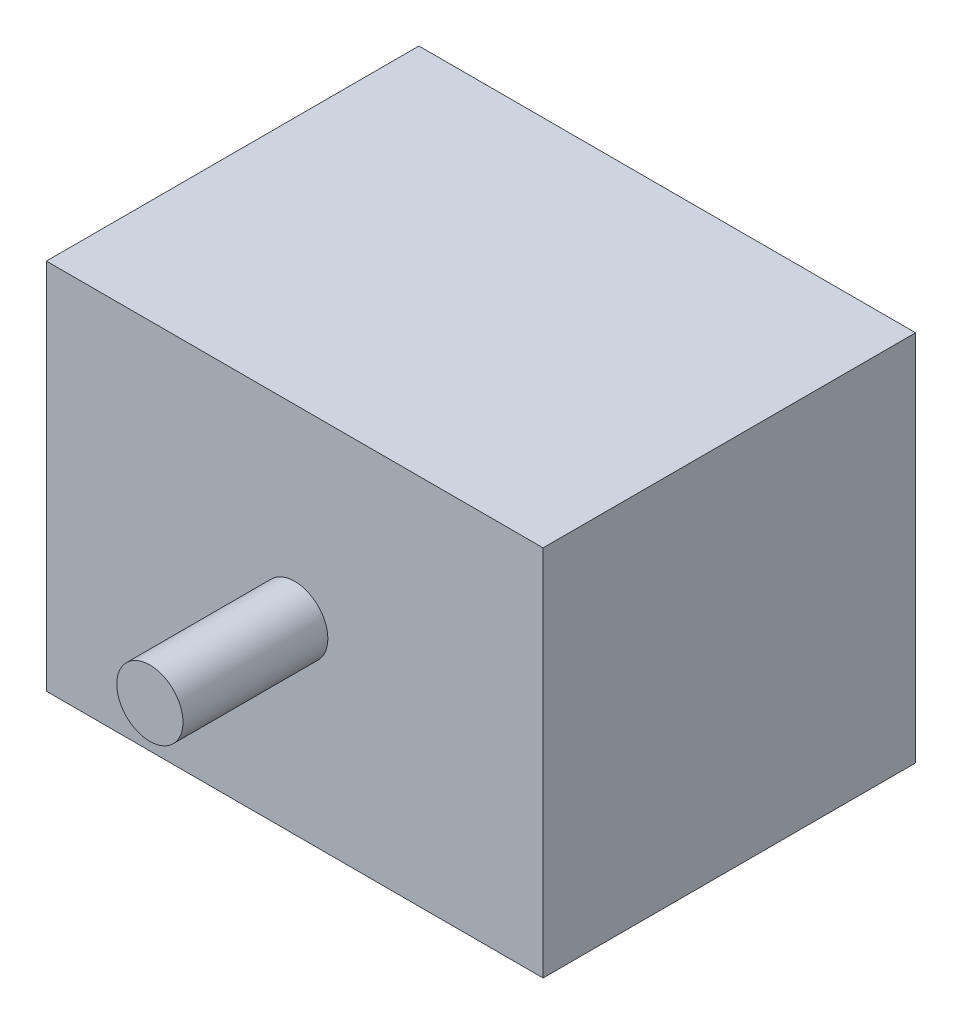
from build123d import *

# Parameters (mm, degrees)
SKETCH_1_W      = 120
SKETCH_1_H      = 90
EXTRUDE_1_DEPTH = 45
SKETCH_2_R      = 8
EXTRUDE_2_DEPTH = 80


with BuildPart() as part:
    # 草图1 → 凸台-拉伸1 (new, symmetric)
    with BuildSketch(Plane.XY):
        Rectangle(SKETCH_1_W, SKETCH_1_H)
    extrude(amount=EXTRUDE_1_DEPTH, both=True)

    # 草图2 → 凸台-拉伸2 (add, symmetric)
    with BuildSketch(Plane.XY):
        Circle(SKETCH_2_R)
    extrude(amount=EXTRUDE_2_DEPTH, both=True)


solid = part.part
